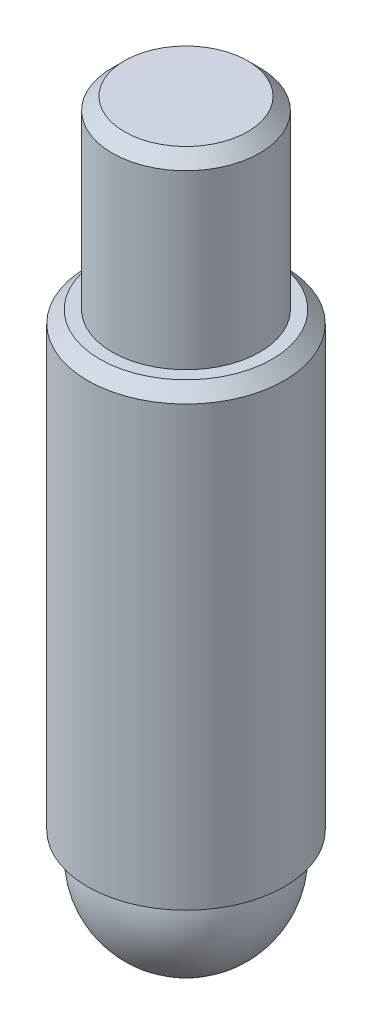
from build123d import *

# Parameters (mm, degrees)
BOSS_EXTRUDE1_DEPTH = 10
SKETCH3_R           = 8
BOSS_EXTRUDE2_DEPTH = 5
SKETCH4_R           = 6
BOSS_EXTRUDE3_DEPTH = 15
CHAMFER1_SIZE       = 1


with BuildPart() as part:
    # Sketch1 → Revolve2 (revolve)
    with BuildSketch(Plane.XY, mode=Mode.PRIVATE) as revolve2_sk:
        with BuildLine():
            Line((-2, 0), (-2, 27))
            Line((-2, 27), (-4, 27))
            Line((-4, 27), (-4, 30))
            Line((-4, 30), (-8, 30))
            Line((-8, 30), (-8, 8.392398037))
            Line((-8, 8.392398037), (-6.75, 8.392398037))
            ThreePointArc((-6.75, 8.392398037), (-6.244894811, 3.375866985), (-2.5, 0))
            Line((-2.5, 0), (-2, 0))
        make_face()
    revolve(revolve2_sk.sketch.rotate(Axis((0, 0, 0), (0, 1, 0)), 270), axis=Axis((0, 0, 0), (0, 1, 0)))

    # Sketch2 → Boss-Extrude1 (add)
    with BuildSketch(Plane(origin=(0, 30, 0), x_dir=(1, 0, 0), z_dir=(0, 1, 0))):
        with BuildLine():
            Line((-4, 6.92820323), (-4, 4.472135955))
            ThreePointArc((-4, 4.472135955), (0, -6), (4, 4.472135955))
            Line((4, 4.472135955), (4, 6.92820323))
            ThreePointArc((4, 6.92820323), (0, -8), (-4, 6.92820323))
        make_face()
    extrude(amount=BOSS_EXTRUDE1_DEPTH)

    # Sketch3 → Boss-Extrude2 (add)
    with BuildSketch(Plane(origin=(0, 40, 0), x_dir=(1, 0, 0), z_dir=(0, 1, 0))):
        with Locations(Location((0, 0, 0), (0, 0, 90))):
            Circle(SKETCH3_R)
    extrude(amount=BOSS_EXTRUDE2_DEPTH)

    # Sketch4 → Boss-Extrude3 (add)
    with BuildSketch(Plane(origin=(0, 45, 0), x_dir=(1, 0, 0), z_dir=(0, 1, 0))):
        with Locations(Location((0, 0, 0), (0, 0, 270))):
            Circle(SKETCH4_R)
    extrude(amount=BOSS_EXTRUDE3_DEPTH)

    # Chamfer1
    chamfer1_edges = [part.edges().sort_by_distance(p)[0] for p in [
        (0, 45, 8),
        (0, 60, -6),
    ]]
    chamfer(chamfer1_edges, length=CHAMFER1_SIZE)


solid = part.part
